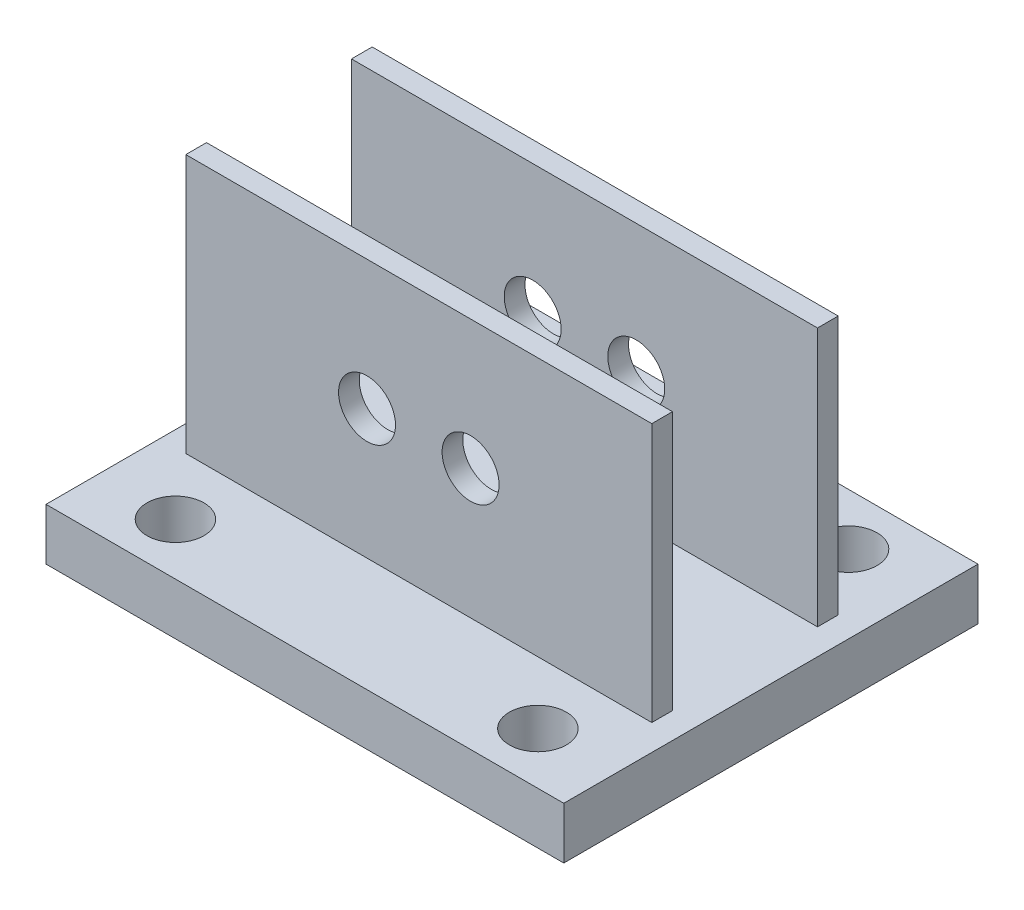
SolidWorks part; units mm, degrees
ref_plane "前视基准面" through (0, 0, 0) normal (0, 0, 1) x (1, 0, 0)
ref_plane "上视基准面" through (0, 0, 0) normal (0, 1, 0) x (1, 0, 0)
ref_plane "右视基准面" through (0, 0, 0) normal (1, 0, 0) x (0, 0, -1)
sketch "草图1" plane through (0, 0, 0) normal (0, 0, 1) x (1, 0, 0)
  line L1 (-45, -25) -> (45, -25)
  line L2 (-45, -25) -> (-45, 25)
  line L3 (-45, 25) -> (45, 25)
  line L4 (45, -25) -> (45, 25)
  line L5 (-45, -25) -> (45, 25) construction
  line L6 (-45, 25) -> (45, -25) construction
  point P0 (0, 0)
  dimension "D1" = 90
  dimension "D2" = 50
extrude "凸台-拉伸1" add sketch "草图1" along normal blind 4
sketch "草图2" plane through (0, 0, 4) normal (0, 0, 1) x (1, 0, 0)
  circle A0 centre (-10, 0) radius 5.5
  circle A1 centre (10, 0) radius 5.5
  dimension "D1" = 11
  dimension "D2" = 11
  dimension "D3" = 20
  dimension "D4" = 10
extrude "切除-拉伸1" cut sketch "草图2" against normal through all
sketch "草图3" plane through (0, -25, 0) normal (0, -1, 0) x (1, 0, 0)
  line L0 (-45, 4) -> (45, 4) construction
  line L1 (-50, -54) -> (50, -54)
  line L2 (-50, -54) -> (-50, 26)
  line L3 (-50, 26) -> (50, 26)
  line L4 (50, -54) -> (50, 26)
  line L5 (-50, -54) -> (50, 26) construction
  line L6 (-50, 26) -> (50, -54) construction
  line L7 (-35, -44) -> (35, -44) construction
  line L8 (-35, -44) -> (-35, 16) construction
  line L9 (-35, 16) -> (35, 16) construction
  line L10 (35, -44) -> (35, 16) construction
  line L11 (-35, -44) -> (35, 16) construction
  line L12 (-35, 16) -> (35, -44) construction
  line L13 (45, 4) -> (45, 0) construction
  circle A0 centre (-35, 16) radius 5.5
  circle A1 centre (35, 16) radius 5.5
  circle A2 centre (35, -44) radius 5.5
  circle A3 centre (-35, -44) radius 5.5
  point P0 (-0.437, -1.836)
  point P6 (0, -14)
  dimension "D5" = 11
  dimension "D6" = 12
  dimension "D1" = 100
  dimension "D2" = 80
  dimension "D3" = 70
  dimension "D4" = 60
  dimension "D7" = 5
extrude "凸台-拉伸2" add sketch "草图3" along normal blind 10
ref_plane "中心面" through (0, 0, -14) normal (0, 0, -1) x (-1, 0, 0)
mirror "镜向1" about plane through (0, 0, -14) normal (0, 0, -1) of "凸台-拉伸1"
sketch "草图4" plane through (0, 0, -28) normal (0, 0, 1) x (1, 0, 0)
  circle A0 centre (-10, 0) radius 5.5
  circle A1 centre (10, 0) radius 5.5
extrude "切除-拉伸2" cut sketch "草图4" against normal through all
ref_plane "基准面1" through (0, 0, -14) normal (0, 0, 1) x (1, 0, 0)
